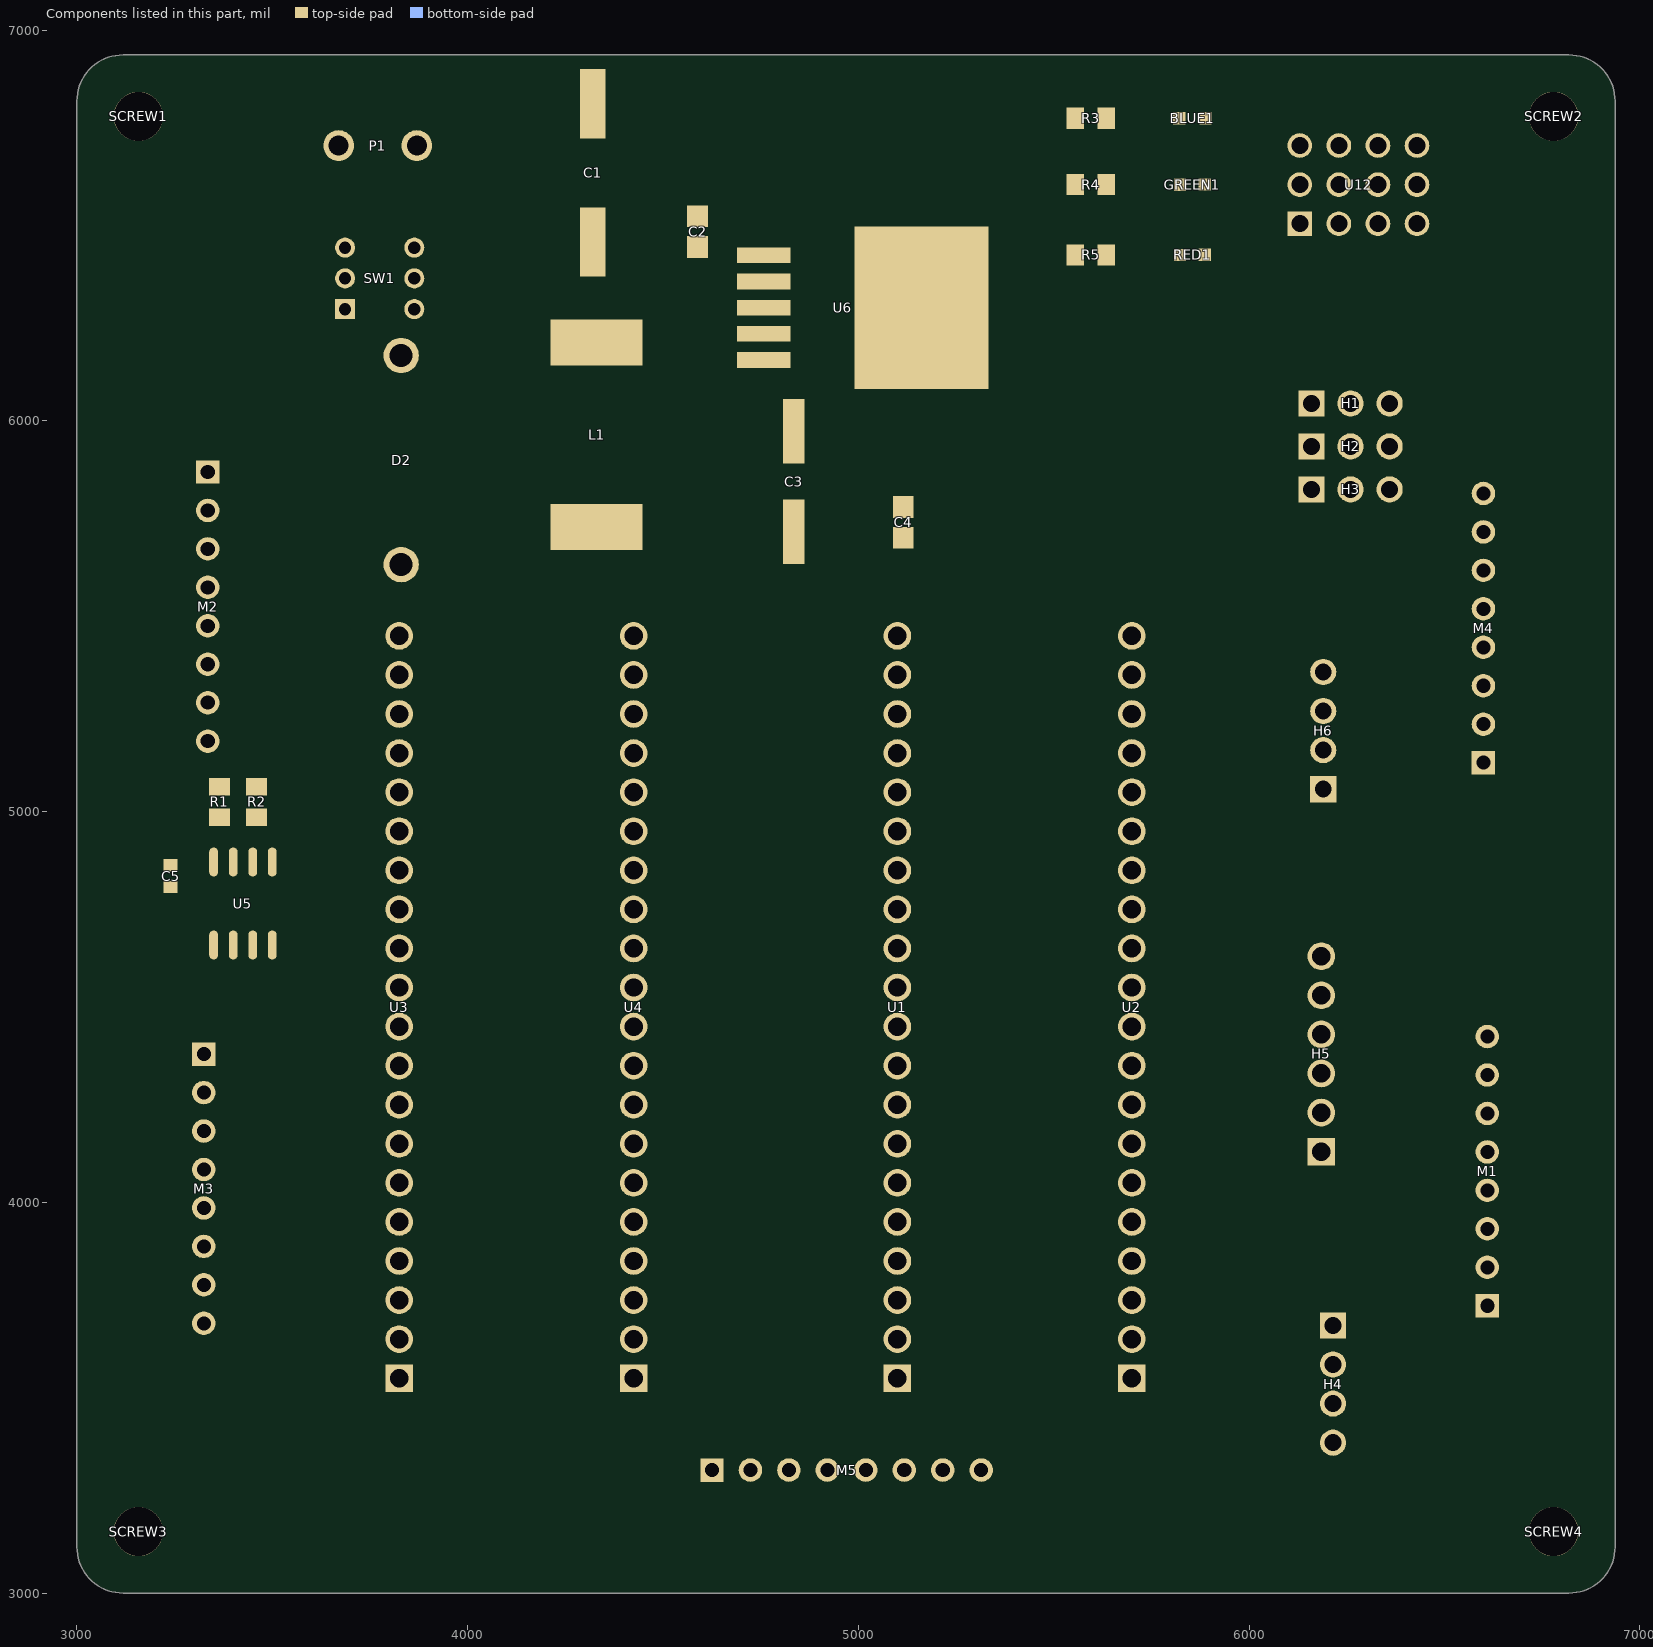
[diagram p0: the components of this part, seen from the top]
# Altium PCB MISC50151.pcbdoc (part 3 of 4)
Units mil, origin at the board's own origin, x right, y up, seen from the top; angles counter-clockwise.
Board outline 3937.01 x 3937.01 mil, 4 copper layers (Top Layer, Inner1, Inner2, Bottom Layer), stack 62.447 mil thick; 39 components, 26 nets, 211 pads, 230 vias.

## Other copper
Top Layer:
  region net $1N596: 3820,6760 3906.42,6760 3939.47,6726.95 3939.47,6444.47 3910,6415 3830,6415 3785,6460 3785,6725
  region net 12.6V: 3820,6395 3980,6395 4135,6550 4395,6550 4475,6470 4815,6470 4830,6455 4830,6415 4820,6405 4420,6405 4355,6340 3823.72,6340 3812.4,6351.32 3812.4,6387.4
  region net $1N570: 4814.09,6380 4837.7,6356.39 4820,6338.69 4820,6335 4640,6335 4450,6145 3902.73,6145 3866.91,6109.18 3785.82,6109.18 3765,6130 3765,6190 3795,6220 3875.2,6220 3930.2,6275 4330,6275 4435,6380
  region net 5V: 4820.41,6244.59 4825,6240 4825,6210 4820,6205 4695,6205 4460,5970 4460,5845 4500,5805 4915,5805 4990,5730 5150,5730 5165,5715 5165,5683.13 5116.87,5635 4225,5635 4185,5675 4185,6055 4220,6090 4445,6090 4599.59,6244.59
  region net $1N591: 5775.75,6765 5775.75,6785 5783.42,6785.36 5791.02,6786.45 5798.49,6788.25 5805.75,6790.75 5805.75,6759.25 5798.49,6761.75 5791.02,6763.55 5783.42,6764.64 5775.75,6765
  region net $1N595: 5792.78,6599.86 5792.78,6609.86 5796.23,6610.18 5799.57,6611.14 5802.68,6612.69 5805.45,6614.79 5807.78,6617.36 5807.78,6592.36 5805.45,6594.94 5802.68,6597.03 5799.57,6598.59 5796.23,6599.54 5792.78,6599.86
  region net 5V: 6270,5999.44 6250,5999.44 6249.66,6001 6248.7,6003.23 6247.21,6005.98 6245.28,6009.12 6243,6012.52 6240.45,6016.04 6237.72,6019.53 6234.9,6022.87 6285.1,6022.87 6282.28,6019.53 6279.55,6016.04 6277,6012.52 6274.72,6009.12 6272.79,6005.98 6271.3,6003.23 6270.34,6001
  region net 5V: 6270,5889.44 6250,5889.44 6249.66,5891 6248.7,5893.23 6247.21,5895.98 6245.28,5899.12 6243,5902.52 6240.45,5906.04 6237.72,5909.53 6234.9,5912.87 6285.1,5912.87 6282.28,5909.53 6279.55,5906.04 6277,5902.52 6274.72,5899.12 6272.79,5895.98 6271.3,5893.23 6270.34,5891
  region net 5V: 6250,5980.56 6270,5980.56 6270.34,5979 6271.3,5976.77 6272.79,5974.02 6274.72,5970.88 6277,5967.48 6279.55,5963.96 6282.28,5960.47 6285.1,5957.13 6234.9,5957.13 6237.72,5960.47 6240.45,5963.96 6243,5967.48 6245.28,5970.88 6247.21,5974.02 6248.7,5976.77 6249.66,5979
  region net 5V: 6270,5779.44 6250,5779.44 6249.66,5781 6248.7,5783.23 6247.21,5785.98 6245.28,5789.12 6243,5792.52 6240.45,5796.04 6237.72,5799.53 6234.9,5802.87 6285.1,5802.87 6282.28,5799.53 6279.55,5796.04 6277,5792.52 6274.72,5789.12 6272.79,5785.98 6271.3,5783.23 6270.34,5781
  region net 5V: 6250,5870.56 6270,5870.56 6270.34,5869 6271.3,5866.77 6272.79,5864.02 6274.72,5860.88 6277,5857.48 6279.55,5853.96 6282.28,5850.47 6285.1,5847.13 6234.9,5847.13 6237.72,5850.47 6240.45,5853.96 6243,5857.48 6245.28,5860.88 6247.21,5864.02 6248.7,5866.77 6249.66,5869
  region net 12.6V: 5488.34,6760 5488.34,6790 5496.18,6790.34 5503.97,6791.37 5511.64,6793.08 5519.12,6795.45 5526.38,6798.47 5533.34,6802.11 5533.34,6747.89 5526.38,6751.53 5519.12,6754.55 5511.64,6756.92 5503.97,6758.63 5496.18,6759.66 5488.34,6760
  region net $1N591: 5686.66,6785 5686.66,6765 5681.71,6764.67 5676.84,6763.69 5672.15,6762.08 5667.71,6759.86 5663.6,6757.07 5659.9,6753.77 5656.66,6750 5656.66,6800 5659.9,6796.23 5663.6,6792.93 5667.71,6790.14 5672.15,6787.92 5676.84,6786.31 5681.71,6785.33 5686.66,6785
  region net 5V: 5545,6662.11 5565,6662.11 5565.38,6656.53 5566.51,6651.05 5568.37,6645.77 5570.92,6640.8 5574.13,6636.22 5577.92,6632.11 5533.34,6632.11 5536.78,6636.37 5539.68,6641.03 5541.98,6646.01 5543.65,6651.24 5544.66,6656.63 5545,6662.11
  region net 5V: 5503.34,6595 5503.34,6615 5508.29,6615.33 5513.16,6616.31 5517.85,6617.92 5522.29,6620.14 5526.4,6622.93 5530.1,6626.23 5533.34,6630 5533.34,6580 5530.1,6583.77 5526.4,6587.07 5522.29,6589.86 5517.85,6592.08 5513.16,6593.69 5508.29,6594.67 5503.34,6595
  region net $1N595: 5671.66,6609.86 5671.66,6599.86 5668.21,6599.54 5664.87,6598.59 5661.76,6597.03 5659,6594.94 5656.66,6592.36 5656.66,6617.36 5659,6614.79 5661.76,6612.69 5664.87,6611.14 5668.21,6610.18 5671.66,6609.86
  region net 3.3V: 5545,6482.11 5565,6482.11 5565.38,6476.53 5566.51,6471.05 5568.37,6465.77 5570.92,6460.8 5574.13,6456.22 5577.92,6452.11 5533.34,6452.11 5536.78,6456.37 5539.68,6461.03 5541.98,6466.01 5543.65,6471.24 5544.66,6476.63 5545,6482.11
  region net $1N953: 5671.66,6430 5671.66,6420 5668.21,6419.68 5664.87,6418.72 5661.76,6417.17 5659,6415.07 5656.66,6412.5 5656.66,6437.5 5659,6434.93 5661.76,6432.83 5664.87,6431.28 5668.21,6430.32 5671.66,6430
  region net $1N953: 5792.77,6420 5792.77,6430 5796.23,6430.32 5799.57,6431.28 5802.68,6432.83 5805.44,6434.93 5807.77,6437.5 5807.77,6412.5 5805.44,6415.07 5802.68,6417.17 5799.57,6418.72 5796.23,6419.68 5792.77,6420
  region net 12.6V: 3828.74,6350 3828.74,6380 3831.3,6380.1 3833.98,6380.36 3839.27,6381.31 3841.67,6381.95 3843.77,6382.66 3845.47,6383.41 3846.65,6384.19 3846.65,6345.81 3845.47,6346.59 3843.77,6347.35 3841.67,6348.06 3839.27,6348.69 3833.98,6349.64 3831.3,6349.91
  region net 12.6V: 4872.07,6438.86 4872.07,6408.86 4860.73,6408.54 4849.42,6407.59 4838.19,6406 4827.07,6403.78 4827.07,6443.94 4838.19,6441.72 4849.42,6440.13 4860.73,6439.18 4872.07,6438.86
  region net M_GYRO_SCL: 5728.87,4793.84 5696.46,4812.11 5693.59,4814.61 5690.44,4816.74 5687.18,4818.59 5683.94,4820.21 5678.12,4823.04 5675.83,4824.39 5674.14,4825.78 5726.95,4827 5725.7,4825.33 5724.63,4823.49 5723.76,4821.51 5723.07,4819.41 5722.57,4817.22 5722.25,4814.95 5722.11,4812.65 5722.16,4810.32 5722.38,4807.99 5722.79,4805.69 5723.37,4803.45 5724.12,4801.28 5725.05,4799.21 5726.15,4797.26 5727.43,4795.47
  region net M_GYRO_SDA: 5737.65,4919.42 5730.58,4912.35 5720.24,4913.16 5697.78,4914.64 5735.36,4952.22 5736.84,4929.76
  region net M_MOTER5_RX: 5128.87,3893.84 5096.46,3912.11 5093.59,3914.61 5090.44,3916.74 5087.18,3918.59 5083.94,3920.21 5078.12,3923.04 5075.83,3924.39 5074.14,3925.78 5126.95,3927 5125.7,3925.33 5124.63,3923.49 5123.76,3921.51 5123.07,3919.41 5122.57,3917.22 5122.25,3914.95 5122.11,3912.65 5122.16,3910.32 5122.38,3907.99 5122.79,3905.69 5123.37,3903.45 5124.12,3901.28 5125.05,3899.21 5126.15,3897.26 5127.43,3895.47
  region net M_MOTER5_TX: 5137.65,4019.42 5130.58,4012.35 5120.24,4013.16 5097.78,4014.64 5135.36,4052.22 5136.84,4029.76
  region net M_SAVE_RX: 5137.65,4719.42 5130.58,4712.35 5120.24,4713.16 5097.78,4714.64 5135.36,4752.22 5136.84,4729.76
  region net M_SLAVE_TX: 5069.42,4812.35 5062.35,4819.42 5063.16,4829.76 5064.64,4852.22 5102.22,4814.64 5079.76,4813.16
  region net S_SAVE_3_RX: 3776.76,3945 3776.76,3955 3784.64,3961.74 3801.56,3976.57 3801.56,3923.43 3784.64,3938.26
  region net S_SAVE_3_RX: 3873.24,3955 3873.24,3945 3865.36,3938.26 3848.44,3923.43 3848.44,3976.57 3865.36,3961.74
  region net S_SAVE_3_TX: 3782.53,4037.93 3771.93,4047.93 3772.69,4048.06 3773.65,4048.46 3776.05,4049.94 3779,4052.25 3782.34,4055.25 3785.93,4058.8 3789.62,4062.76 3793.27,4066.99 3796.73,4071.36 3807.34,4019.28 3806.28,4020 3805.13,4020.97 3802.59,4023.5 3796.64,4029.77 3793.32,4032.84 3791.6,4034.23 3789.84,4035.45 3788.05,4036.47 3786.23,4037.25 3784.39,4037.75
  region net S_SAVE_3_TX: 3873.24,4055 3873.24,4045 3865.36,4038.26 3848.44,4023.43 3848.44,4076.57 3865.36,4061.74
  region net S_485_EN: 3787.35,4180.58 3794.42,4187.65 3804.76,4186.84 3827.22,4185.36 3789.64,4147.78 3788.16,4170.24
  region net M_SLAVE_TX: 3787.35,4780.58 3794.42,4787.65 3804.76,4786.84 3827.22,4785.36 3789.64,4747.78 3788.16,4770.24
  region net S_SAVE_2_TX: 3873.24,4855 3873.24,4845 3865.36,4838.26 3848.44,4823.43 3848.44,4876.57 3865.36,4861.74
  region net BUS_S_A: 6635.34,4358.48 6642.42,4351.4 6641.97,4348.84 6641.34,4342.59 6639.94,4324.18 6608.12,4356 6626.53,4357.4 6632.78,4358.03
  region net BUS_S_B: 6584.66,4392.07 6577.58,4399.15 6578.03,4401.71 6578.66,4407.96 6580.06,4426.37 6611.88,4394.55 6593.47,4393.15 6587.22,4392.52
  region net 12.6V: 3410,5884.49 3410,5854.49 3403.12,5854.17 3396.29,5853.23 3389.58,5851.66 3383.04,5849.48 3376.73,5846.71 3370.7,5843.37 3365,5839.49 3365,5899.49 3370.7,5895.61 3376.73,5892.27 3383.04,5889.5 3389.58,5887.32 3396.29,5885.75 3403.12,5884.81
  region net BUS_S_A: 3367.42,5253.6 3360.34,5246.52 3357.78,5246.97 3351.53,5247.6 3333.12,5249 3364.94,5280.82 3366.34,5262.41 3366.97,5256.16
  region net BUS_S_B: 3313.54,5151.97 3306.46,5159.05 3307.17,5159.98 3307.65,5161.12 3307.94,5162.43 3308.05,5163.89 3307.87,5167.13 3307.3,5170.61 3305.77,5177.39 3305.22,5180.23 3305.06,5182.39 3336.88,5150.57 3334.72,5150.73 3331.88,5151.28 3325.1,5152.81 3321.62,5153.38 3318.38,5153.56 3316.92,5153.45 3315.61,5153.16 3314.47,5152.68
  region net BUS_S_A: 6559.16,5711.06 6559.16,5721.06 6561.29,5722.56 6566.15,5726.53 6580.16,5738.56 6580.16,5693.56 6566.15,5705.59 6561.29,5709.56
  region net BUS_S_A: 6632.42,5690.72 6625.34,5683.64 6622.78,5684.09 6616.53,5684.72 6598.12,5686.12 6629.94,5717.94 6631.34,5699.53 6631.97,5693.28
  region net M_MOTER5_RX: 5183.64,3340.34 5190.72,3347.42 5193.28,3346.97 5199.53,3346.34 5217.94,3344.94 5186.12,3313.12 5184.72,3331.53 5184.09,3337.78
  region net M_MOTER5_TX: 5282.07,3340.34 5289.15,3347.42 5291.71,3346.97 5297.96,3346.34 5316.37,3344.94 5284.55,3313.12 5283.15,3331.53 5282.52,3337.78
  region net BUS_S_A: 3292.58,3814.28 3299.66,3821.36 3302.22,3820.91 3308.47,3820.28 3326.88,3818.88 3295.06,3787.06 3293.66,3805.47 3293.03,3811.72
  region net BUS_S_B: 3330,3649.67 3320,3649.67 3318.5,3651.8 3314.53,3656.66 3302.5,3670.67 3347.5,3670.67 3335.47,3656.66 3331.5,3651.8
  region net BUS_S_B: 3284.16,3685.51 3284.16,3695.51 3286.29,3697.01 3291.15,3700.98 3305.16,3713.01 3305.16,3668.01 3291.15,3680.04 3286.29,3684.01
  region net M_GYRO_SCL: 6179.25,3613.68 6186.32,3620.75 6189.09,3620.42 6196.11,3619.85 6217.1,3618.4 6181.6,3582.9 6180.15,3603.89 6179.58,3610.91
  region net M_GYRO_SDA: 6210,3522.14 6220,3522.14 6220.19,3521.02 6220.73,3519.93 6221.57,3518.85 6222.67,3517.79 6225.48,3515.75 6228.8,3513.8 6235.56,3510.22 6238.28,3508.61 6239.33,3507.86 6240.1,3507.13 6189.9,3507.13 6190.67,3507.86 6191.72,3508.61 6194.44,3510.22 6201.2,3513.8 6204.52,3515.75 6207.33,3517.79 6208.43,3518.85 6209.27,3519.93 6209.81,3521.02
  region net M_SAVE_RX: 6136.76,4425 6136.76,4435 6144.64,4441.74 6161.56,4456.57 6161.56,4403.42 6144.64,4418.26
  region net S_SAVE_2_TX: 6136.76,4325 6136.76,4335 6144.64,4341.74 6161.56,4356.57 6161.56,4303.42 6144.64,4318.26
  region net S_SAVE_3_RX: 6222.08,4195.88 6211.92,4191.9 6210.48,4193.07 6208.79,4194 6206.91,4194.7 6204.85,4195.2 6202.67,4195.52 6200.38,4195.7 6195.66,4195.7 6190.97,4195.42 6186.59,4195.06 6182.81,4194.83 6179.89,4194.94 6220.43,4229.31 6220.4,4217.67 6220.72,4207.18 6221.3,4199.39 6221.67,4197.01
  region net S_SAVE_3_TX: 6144.26,4163.66 6151.33,4170.74 6154.94,4168.46 6158.86,4166.79 6163,4165.77 6167.24,4165.43 6149.57,4147.75 6149.22,4152 6148.21,4156.14 6146.54,4160.06 6144.26,4163.66
  region net 3.3V: 6172.88,6615 6172.88,6595 6171.3,6594.69 6169.13,6593.83 6166.49,6592.49 6163.51,6590.74 6160.33,6588.68 6157.07,6586.38 6153.86,6583.92 6150.83,6581.38 6150.83,6628.62 6153.86,6626.08 6157.07,6623.62 6160.33,6621.32 6163.51,6619.26 6166.49,6617.51 6169.13,6616.17 6171.3,6615.31
  region net 3.3V: 6106.75,6567.61 6092.61,6581.75 6093.51,6583.08 6094.43,6585.23 6095.35,6588.05 6096.22,6591.38 6097.01,6595.09 6097.69,6599.02 6098.22,6603.03 6098.57,6606.97 6131.97,6573.57 6128.03,6573.22 6124.02,6572.69 6120.09,6572.01 6116.38,6571.22 6113.05,6570.35 6110.23,6569.43 6108.08,6568.51
  region net 5V: 6087.12,6695 6087.12,6715 6088.7,6715.31 6090.87,6716.17 6093.51,6717.51 6096.49,6719.26 6099.67,6721.32 6102.93,6723.62 6106.14,6726.08 6109.17,6728.62 6109.17,6681.38 6106.14,6683.92 6102.93,6686.38 6099.67,6688.68 6096.49,6690.74 6093.51,6692.49 6090.87,6693.83 6088.7,6694.69
  region net 5V: 6172.88,6715 6172.88,6695 6171.3,6694.69 6169.13,6693.83 6166.49,6692.49 6163.51,6690.74 6160.33,6688.68 6157.07,6686.38 6153.86,6683.92 6150.83,6681.38 6150.83,6728.62 6153.86,6726.08 6157.07,6723.62 6160.33,6721.32 6163.51,6719.26 6166.49,6717.51 6169.13,6716.17 6171.3,6715.31
  region net 3.3V: 6187.12,6595 6187.12,6615 6188.7,6615.31 6190.87,6616.17 6193.51,6617.51 6196.49,6619.26 6199.67,6621.32 6202.93,6623.62 6206.14,6626.08 6209.17,6628.62 6209.17,6581.38 6206.14,6583.92 6202.93,6586.38 6199.67,6588.68 6196.49,6590.74 6193.51,6592.49 6190.87,6593.83 6188.7,6594.69
  region net 3.3V: 6272.88,6615 6272.88,6595 6271.3,6594.69 6269.13,6593.83 6266.49,6592.49 6263.51,6590.74 6260.33,6588.68 6257.07,6586.38 6253.86,6583.92 6250.83,6581.38 6250.83,6628.62 6253.86,6626.08 6257.07,6623.62 6260.33,6621.32 6263.51,6619.26 6266.49,6617.51 6269.13,6616.17 6271.3,6615.31
  region net 5V: 6187.12,6695 6187.12,6715 6188.7,6715.31 6190.87,6716.17 6193.51,6717.51 6196.49,6719.26 6199.67,6721.32 6202.93,6723.62 6206.14,6726.08 6209.17,6728.62 6209.17,6681.38 6206.14,6683.92 6202.93,6686.38 6199.67,6688.68 6196.49,6690.74 6193.51,6692.49 6190.87,6693.83 6188.7,6694.69
  region net 5V: 6272.88,6715 6272.88,6695 6271.3,6694.69 6269.13,6693.83 6266.49,6692.49 6263.51,6690.74 6260.33,6688.68 6257.07,6686.38 6253.86,6683.92 6250.83,6681.38 6250.83,6728.62 6253.86,6726.08 6257.07,6723.62 6260.33,6721.32 6263.51,6719.26 6266.49,6717.51 6269.13,6716.17 6271.3,6715.31
  region net 3.3V: 6372.88,6615 6372.88,6595 6371.3,6594.69 6369.13,6593.83 6366.49,6592.49 6363.51,6590.74 6360.33,6588.68 6357.07,6586.38 6353.86,6583.92 6350.83,6581.38 6350.83,6628.62 6353.86,6626.08 6357.07,6623.62 6360.33,6621.32 6363.51,6619.26 6366.49,6617.51 6369.13,6616.17 6371.3,6615.31
  region net 3.3V: 6287.12,6595 6287.12,6615 6288.7,6615.31 6290.87,6616.17 6293.51,6617.51 6296.49,6619.26 6299.67,6621.32 6302.93,6623.62 6306.14,6626.08 6309.17,6628.62 6309.17,6581.38 6306.14,6583.92 6302.93,6586.38 6299.67,6588.68 6296.49,6590.74 6293.51,6592.49 6290.87,6593.83 6288.7,6594.69
  region net 5V: 6372.88,6715 6372.88,6695 6371.3,6694.69 6369.13,6693.83 6366.49,6692.49 6363.51,6690.74 6360.33,6688.68 6357.07,6686.38 6353.86,6683.92 6350.83,6681.38 6350.83,6728.62 6353.86,6726.08 6357.07,6723.62 6360.33,6721.32 6363.51,6719.26 6366.49,6717.51 6369.13,6716.17 6371.3,6715.31
  region net 5V: 6287.12,6695 6287.12,6715 6288.7,6715.31 6290.87,6716.17 6293.51,6717.51 6296.49,6719.26 6299.67,6721.32 6302.93,6723.62 6306.14,6726.08 6309.17,6728.62 6309.17,6681.38 6306.14,6683.92 6302.93,6686.38 6299.67,6688.68 6296.49,6690.74 6293.51,6692.49 6290.87,6693.83 6288.7,6694.69
  region net 3.3V: 6472.88,6615 6472.88,6595 6471.3,6594.69 6469.13,6593.83 6466.49,6592.49 6463.51,6590.74 6460.33,6588.68 6457.07,6586.38 6453.86,6583.92 6450.83,6581.38 6450.83,6628.62 6453.86,6626.08 6457.07,6623.62 6460.33,6621.32 6463.51,6619.26 6466.49,6617.51 6469.13,6616.17 6471.3,6615.31
  region net 3.3V: 6387.12,6595 6387.12,6615 6388.7,6615.31 6390.87,6616.17 6393.51,6617.51 6396.49,6619.26 6399.67,6621.32 6402.93,6623.62 6406.14,6626.08 6409.17,6628.62 6409.17,6581.38 6406.14,6583.92 6402.93,6586.38 6399.67,6588.68 6396.49,6590.74 6393.51,6592.49 6390.87,6593.83 6388.7,6594.69
  region net 5V: 6387.12,6695 6387.12,6715 6388.7,6715.31 6390.87,6716.17 6393.51,6717.51 6396.49,6719.26 6399.67,6721.32 6402.93,6723.62 6406.14,6726.08 6409.17,6728.62 6409.17,6681.38 6406.14,6683.92 6402.93,6686.38 6399.67,6688.68 6396.49,6690.74 6393.51,6692.49 6390.87,6693.83 6388.7,6694.69
  region net S_SAVE_3_RX: 3355,4617.87 3345,4617.87 3344.73,4620.11 3344.02,4622.29 3343.01,4624.4 3341.85,4626.4 3339.69,4630 3338.97,4631.54 3338.7,4632.87 3361.3,4632.87 3361.03,4631.54 3360.31,4630 3358.15,4626.4 3356.99,4624.4 3355.98,4622.29 3355.27,4620.11
  region net S_485_EN: 3395,4699.61 3405,4699.61 3405.27,4697.37 3405.98,4695.19 3406.99,4693.08 3408.15,4691.08 3410.31,4687.48 3411.03,4685.94 3411.3,4684.61 3388.7,4684.61 3388.97,4685.94 3389.69,4687.48 3391.85,4691.08 3393.01,4693.08 3394.02,4695.19 3394.73,4697.37
  region net S_485_EN: 3445,4699.61 3455,4699.61 3455.27,4697.37 3455.98,4695.19 3456.99,4693.08 3458.15,4691.08 3460.31,4687.48 3461.03,4685.94 3461.3,4684.61 3438.7,4684.61 3438.97,4685.94 3439.69,4687.48 3441.85,4691.08 3443.01,4693.08 3444.02,4695.19 3444.73,4697.37
  region net S_SAVE_3_TX: 3505,4617.87 3495,4617.87 3494.73,4620.11 3494.02,4622.29 3493.01,4624.4 3491.85,4626.4 3489.69,4630 3488.97,4631.54 3488.7,4632.87 3511.3,4632.87 3511.03,4631.54 3510.31,4630 3508.15,4626.4 3506.99,4624.4 3505.98,4622.29 3505.27,4620.11
  region net 3.3V: 3308.7,4852.56 3308.7,4872.56 3311.51,4872.65 3314.3,4872.9 3317.04,4873.3 3319.72,4873.85 3324.78,4875.33 3327.13,4876.24 3329.33,4877.25 3331.34,4878.34 3333.16,4879.52 3334.76,4880.76 3336.12,4882.05 3337.22,4883.39 3338.03,4884.76 3338.53,4886.16 3338.7,4887.56 3338.7,4845.39 3338.53,4846.06 3338.03,4846.73 3337.22,4847.39 3336.12,4848.02 3333.16,4849.24 3329.33,4850.32 3324.78,4851.24 3319.72,4851.94 3314.3,4852.4
  region net BUS_S_B: 3395,4912.13 3405,4912.13 3405.27,4909.89 3405.98,4907.71 3406.99,4905.6 3408.15,4903.6 3410.31,4900 3411.03,4898.46 3411.3,4897.13 3388.7,4897.13 3388.97,4898.46 3389.69,4900 3391.85,4903.6 3393.01,4905.6 3394.02,4907.71 3394.73,4909.89
  region net BUS_S_B: 3403.54,4831.46 3384.11,4826.18 3385.44,4827.76 3386.62,4829.66 3387.64,4831.78 3388.45,4834.03 3389.04,4836.31 3389.36,4838.53 3389.39,4840.58 3389.11,4842.39 3411.3,4845.39 3411.12,4844.07 3410.63,4842.46 3409.87,4840.65 3408.87,4838.73 3406.39,4834.85 3404.98,4833.05
  region net BUS_S_A: 3453.54,4831.46 3434.11,4826.18 3435.44,4827.76 3436.62,4829.66 3437.64,4831.78 3438.45,4834.03 3439.04,4836.31 3439.36,4838.53 3439.39,4840.58 3439.11,4842.39 3461.3,4845.39 3461.12,4844.07 3460.63,4842.46 3459.87,4840.65 3458.87,4838.73 3456.39,4834.85 3454.98,4833.05
  region net BUS_S_A: 3445,4912.13 3455,4912.13 3455.27,4909.89 3455.98,4907.71 3456.99,4905.6 3458.15,4903.6 3460.31,4900 3461.03,4898.46 3461.3,4897.13 3438.7,4897.13 3438.97,4898.46 3439.69,4900 3441.85,4903.6 3443.01,4905.6 3444.02,4907.71 3444.73,4909.89
  region net 3.3V: 3230,4908.31 3250,4908.31 3250.32,4902.06 3251.26,4895.87 3252.82,4889.81 3254.98,4883.93 3257.72,4878.31 3222.28,4878.31 3225.02,4883.93 3227.18,4889.81 3228.74,4895.87 3229.68,4902.06 3230,4908.31
  region net 3.3V: 3287.72,4872.56 3287.72,4852.56 3280.05,4852.2 3272.44,4851.11 3264.98,4849.31 3257.72,4846.81 3257.72,4878.31 3264.98,4875.81 3272.44,4874.01 3280.05,4872.92 3287.72,4872.56
  region net BUS_S_B: 3397.41,4960.29 3385.53,4958.03 3381.92,4960.31 3378,4961.98 3373.86,4962.99 3369.62,4963.34 3392.11,4976.2 3392.45,4971.95 3393.47,4967.82 3395.14,4963.89 3397.41,4960.29
  region net BUS_S_B: 3332.59,5010.97 3344.47,5013.23 3348.08,5010.95 3352,5009.28 3356.14,5008.27 3360.38,5007.92 3337.89,4995.06 3337.55,4999.31 3336.53,5003.44 3334.86,5007.37 3332.59,5010.97
  region net 3.3V: 3450,5116.66 3470,5116.66 3470.33,5111.71 3471.31,5106.84 3472.92,5102.15 3475.14,5097.71 3477.93,5093.6 3481.23,5089.9 3485,5086.66 3435,5086.66 3438.77,5089.9 3442.07,5093.6 3444.86,5097.71 3447.08,5102.15 3448.69,5106.84 3449.67,5111.71 3450,5116.66
  region net BUS_S_A: 3455,4948.34 3445,4948.34 3444.68,4951.79 3443.72,4955.13 3442.17,4958.24 3440.07,4961 3437.5,4963.34 3462.5,4963.34 3459.93,4961 3457.83,4958.24 3456.28,4955.13 3455.32,4951.79 3455,4948.34
  region net BUS_S_A: 3492.41,4960.29 3480.53,4958.03 3476.92,4960.31 3473,4961.98 3468.86,4962.99 3464.62,4963.34 3487.11,4976.2 3487.45,4971.95 3488.47,4967.82 3490.14,4963.89 3492.41,4960.29
  region net BUS_S_A: 3427.59,5010.97 3439.47,5013.23 3443.08,5010.95 3447,5009.28 3451.14,5008.27 3455.38,5007.92 3432.89,4995.06 3432.55,4999.31 3431.53,5003.44 3429.86,5007.37 3427.59,5010.97
  region net 3.3V: 6530,6159.41 6550,6159.41 6550.09,6157.25 6550.31,6155.14 6551,6151.13 6551.69,6147.67 6552.01,6145 6527.99,6145 6528.31,6147.67 6529,6151.13 6529.69,6155.14 6529.91,6157.25
  region net 3.3V: 3470,5160.59 3450,5160.59 3449.91,5162.75 3449.69,5164.86 3449,5168.87 3448.31,5172.33 3447.99,5175 3472.01,5175 3471.69,5172.33 3471,5168.87 3470.31,5164.86 3470.09,5162.75
  region net 3.3V: 3250,4900.59 3230,4900.59 3229.91,4902.75 3229.69,4904.86 3229,4908.87 3228.31,4912.33 3227.99,4915 3252.01,4915 3251.69,4912.33 3251,4908.87 3250.31,4904.86 3250.09,4902.75
  region net S_485_EN: 3455,4730 3455.29,4735.35 3456.15,4740.64 3457.57,4745.81 3459.53,4750.8 3462.02,4755.55 3465,4760 3450,4765 3435,4760 3437.98,4755.55 3440.47,4750.8 3442.43,4745.81 3443.85,4740.64 3444.71,4735.35 3445,4730
Inner2:
  region net 3.3V: 5690,5498.24 5710,5498.24 5710.37,5496.7 5711.42,5494.42 5713.06,5491.55 5715.18,5488.24 5720.49,5480.85 5723.48,5477.08 5726.57,5473.44 5673.43,5473.44 5676.52,5477.08 5679.51,5480.85 5684.82,5488.24 5686.94,5491.55 5688.58,5494.42 5689.63,5496.7
  region net 3.3V: 4376.76,5440 4376.76,5460 4378.3,5460.37 4380.58,5461.42 4383.45,5463.06 4386.76,5465.18 4394.15,5470.49 4397.92,5473.48 4401.56,5476.57 4401.56,5423.43 4397.92,5426.52 4394.15,5429.51 4386.76,5434.82 4383.45,5436.94 4380.58,5438.58 4378.3,5439.63
  region net 3.3V: 4383.82,5477.04 4397.96,5491.18 4399.31,5490.35 4401.67,5489.49 4404.85,5488.61 4408.7,5487.77 4417.67,5486.3 4422.46,5485.75 4427.22,5485.36 4389.64,5447.78 4389.25,5452.54 4388.7,5457.33 4387.23,5466.3 4386.39,5470.15 4385.51,5473.33 4384.65,5475.69
  region net 3.3V: 4452.04,5491.18 4466.18,5477.04 4465.35,5475.69 4464.49,5473.33 4463.61,5470.15 4462.77,5466.3 4461.3,5457.33 4460.75,5452.54 4460.36,5447.78 4422.78,5485.36 4427.54,5485.75 4432.33,5486.3 4441.3,5487.77 4445.15,5488.61 4448.33,5489.49 4450.69,5490.35
  region net 3.3V: 5148.24,3760 5148.24,3740 5146.7,3739.63 5144.42,3738.58 5141.55,3736.94 5138.24,3734.82 5130.85,3729.51 5127.08,3726.52 5123.44,3723.43 5123.44,3776.57 5127.08,3773.48 5130.85,3770.49 5138.24,3765.18 5141.55,3763.06 5144.42,3761.42 5146.7,3760.37
  region net 3.3V: 3852.04,3791.18 3866.18,3777.04 3865.35,3775.69 3864.49,3773.33 3863.61,3770.15 3862.77,3766.3 3861.3,3757.33 3860.75,3752.54 3860.36,3747.78 3822.78,3785.36 3827.54,3785.75 3832.33,3786.3 3841.3,3787.77 3845.15,3788.61 3848.33,3789.49 3850.69,3790.35
  region net 12.6V: 3310.3,5823.58 3289.09,5844.79 3293.2,5850.84 3296.74,5857.23 3299.68,5863.93 3301.99,5870.86 3303.66,5877.98 3304.66,5885.22 3305,5892.52 3358.03,5839.49 3350.73,5839.15 3343.49,5838.15 3336.37,5836.48 3329.44,5834.17 3322.74,5831.23 3316.35,5827.69 3310.3,5823.58
  region net 12.6V: 4550.51,3300 4550.51,3330 4557.39,3330.32 4564.22,3331.26 4570.93,3332.83 4577.47,3335.01 4583.78,3337.78 4589.81,3341.12 4595.51,3345 4595.51,3285 4589.81,3288.88 4583.78,3292.22 4577.47,3294.99 4570.93,3297.17 4564.22,3298.74 4557.39,3299.68 4550.51,3300
  region net 12.6V: 3250,4364.49 3250,4394.49 3256.88,4394.81 3263.71,4395.75 3270.42,4397.32 3276.96,4399.5 3283.27,4402.27 3289.3,4405.61 3295,4409.49 3295,4349.49 3289.3,4353.37 3283.27,4356.71 3276.96,4359.48 3270.42,4361.66 3263.71,4363.23 3256.88,4364.17
  region net 3.3V: 6144.44,5147.57 6144.44,5167.57 6146,5167.91 6148.23,5168.86 6150.98,5170.35 6154.12,5172.28 6157.52,5174.57 6161.04,5177.12 6164.53,5179.85 6167.87,5182.67 6167.87,5132.47 6164.53,5135.28 6161.04,5138.01 6157.52,5140.56 6154.12,5142.85 6150.98,5144.78 6148.23,5146.27 6146,5147.23
  region net 3.3V: 6536.88,6127.74 6522.74,6141.88 6524.2,6143.47 6525.54,6145.13 6527.88,6148.44 6529.84,6151.38 6531.51,6153.49 6548.49,6136.51 6546.38,6134.84 6543.44,6132.88 6540.13,6130.54 6538.47,6129.2
  region net 3.3V: 3470,5160.59 3450,5160.59 3449.91,5162.75 3449.69,5164.86 3449,5168.87 3448.31,5172.33 3447.99,5175 3472.01,5175 3471.69,5172.33 3471,5168.87 3470.31,5164.86 3470.09,5162.75
  region net 3.3V: 3450,5189.41 3470,5189.41 3470.09,5187.25 3470.31,5185.14 3471,5181.13 3471.69,5177.67 3472.01,5175 3447.99,5175 3448.31,5177.67 3449,5181.13 3449.69,5185.14 3449.91,5187.25
  region net 3.3V: 3243.12,4932.26 3257.26,4918.12 3255.8,4916.53 3254.46,4914.87 3252.12,4911.56 3250.16,4908.62 3248.49,4906.51 3231.51,4923.49 3233.62,4925.16 3236.56,4927.12 3239.87,4929.46 3241.53,4930.8
  region net 3.3V: 6035,5500 6034.68,5508.04 6033.71,5516.02 6032.1,5523.9 6029.87,5531.62 6027.02,5539.14 6023.58,5546.41 6019.56,5553.38 6015,5560 6045,5570 6075,5560 6070.44,5553.38 6066.42,5546.41 6062.98,5539.14 6060.13,5531.62 6057.9,5523.9 6056.29,5516.02 6055.32,5508.04 6055,5500
  region net 3.3V: 5690,5500 5689.68,5508.04 5688.71,5516.02 5687.1,5523.9 5684.87,5531.62 5682.02,5539.14 5678.58,5546.41 5674.56,5553.38 5670,5560 5697.5,5570 5730,5560 5725.44,5553.38 5721.42,5546.41 5717.98,5539.14 5715.13,5531.62 5712.9,5523.9 5711.29,5516.02 5710.32,5508.04 5710,5500
  region net 3.3V: 5270,5500 5270.32,5508.04 5271.29,5516.02 5272.9,5523.9 5275.13,5531.62 5277.98,5539.14 5281.42,5546.41 5285.44,5553.38 5290,5560 5260,5570 5230,5560 5234.56,5553.38 5238.58,5546.41 5242.02,5539.14 5244.87,5531.62 5247.1,5523.9 5248.71,5516.02 5249.68,5508.04 5250,5500